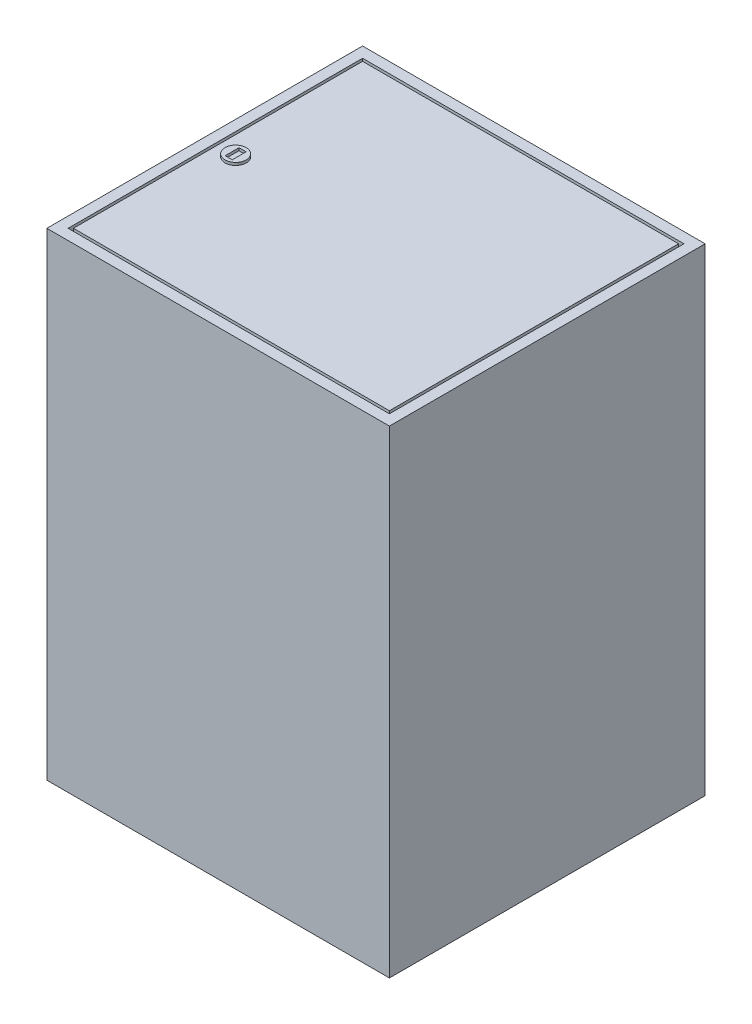
from build123d import *

# Parameters (mm, degrees)
SKETCH_1_W          = 645
SKETCH_1_H          = 900
EXTRUDE_1_DEPTH     = 594.5
SKETCH_2_W          = 605
SKETCH_2_H          = 554.5
SKETCH_2_W_2        = 595
SKETCH_2_H_2        = 544.5
CUT_EXTRUDE_1_DEPTH = 10
SKETCH_3_R          = 20
EXTRUDE_2_DEPTH     = 5
SKETCH_4_W          = 9.930578971
SKETCH_4_H          = 24.659600502
CUT_EXTRUDE_2_DEPTH = 5
SKETCH_5_W          = 605
SKETCH_5_H          = 554.5
SKETCH_5_W_2        = 595
SKETCH_5_H_2        = 544.5
CUT_EXTRUDE_3_DEPTH = 10
SKETCH_6_R          = 20
EXTRUDE_3_DEPTH     = 5
SKETCH_7_W          = 13.385113247
SKETCH_7_H          = 26.065674485
CUT_EXTRUDE_4_DEPTH = 5


with BuildPart() as part:
    # 草图1 → 凸台-拉伸1 (new body)
    with BuildSketch(Plane.XY):
        Rectangle(SKETCH_1_W, SKETCH_1_H)
    extrude(amount=EXTRUDE_1_DEPTH)

    # 草图2 → 切除-拉伸1 (cut)
    with BuildSketch(Plane.XZ.offset(450)):
        with Locations((0, 297.25)):
            Rectangle(SKETCH_2_W, SKETCH_2_H)
        with Locations((0, 297.25)):
            Rectangle(SKETCH_2_W_2, SKETCH_2_H_2, mode=Mode.SUBTRACT)
    extrude(amount=-CUT_EXTRUDE_1_DEPTH, mode=Mode.SUBTRACT)

    # 草图3 → 凸台-拉伸2 (add)
    with BuildSketch(Plane.XZ.offset(450)):
        with Locations(Location((263.592324158, 304.229859051, 0), (0, 0, 90))):
            Circle(SKETCH_3_R)
    extrude(amount=EXTRUDE_2_DEPTH)

    # 草图4 → 切除-拉伸2 (cut)
    with BuildSketch(Plane.XZ.offset(455)):
        with Locations((263.592324158, 304.229859051)):
            Rectangle(SKETCH_4_W, SKETCH_4_H)
    extrude(amount=-CUT_EXTRUDE_2_DEPTH, mode=Mode.SUBTRACT)

    # 草图5 → 切除-拉伸3 (cut)
    with BuildSketch(Plane(origin=(0, 450, 0), x_dir=(1, 0, 0), z_dir=(0, 1, 0))):
        with Locations((0, -297.25)):
            Rectangle(SKETCH_5_W, SKETCH_5_H)
        with Locations((0, -297.25)):
            Rectangle(SKETCH_5_W_2, SKETCH_5_H_2, mode=Mode.SUBTRACT)
    extrude(amount=-CUT_EXTRUDE_3_DEPTH, mode=Mode.SUBTRACT)

    # 草图6 → 凸台-拉伸3 (add)
    with BuildSketch(Plane(origin=(0, 450, 0), x_dir=(1, 0, 0), z_dir=(0, 1, 0))):
        with Locations(Location((-261.325922866, -300.206175598, 0), (0, 0, 90))):
            Circle(SKETCH_6_R)
    extrude(amount=EXTRUDE_3_DEPTH)

    # 草图7 → 切除-拉伸4 (cut)
    with BuildSketch(Plane(origin=(0, 455, 0), x_dir=(1, 0, 0), z_dir=(0, 1, 0))):
        with Locations((-261.325922867, -300.206175599)):
            Rectangle(SKETCH_7_W, SKETCH_7_H)
    extrude(amount=-CUT_EXTRUDE_4_DEPTH, mode=Mode.SUBTRACT)


solid = part.part
